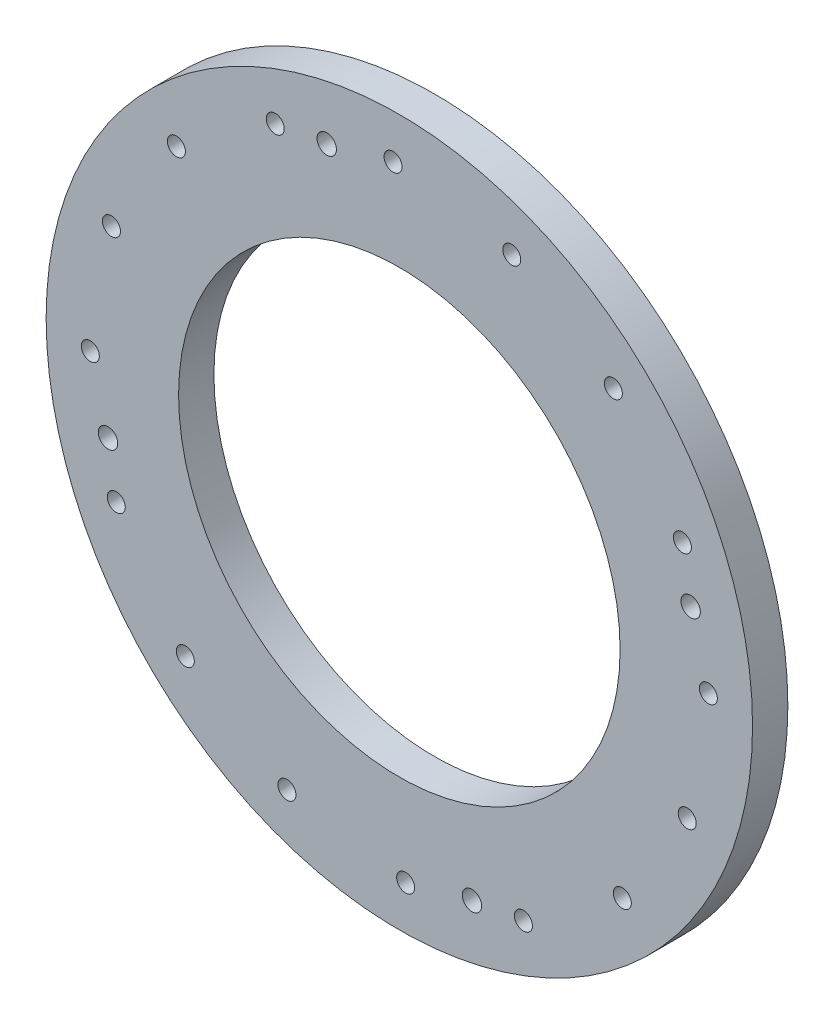
from build123d import *

# Parameters (mm, degrees)
SKETCH_1_R                = 200
EXTRUDE_1_DEPTH           = 10
SKETCH_2_R                = 125
CUT_EXTRUDE_1_DEPTH       = 284.548937575
HOLE_WIZARD_M12_1_D       = 10.2
PATTERN_CIRCULAR_1_COUNT  = 16
HOLE_WIZARD_1_D           = 11
HOLE_WIZARD_1_CBORE_D     = 18
HOLE_WIZARD_1_CBORE_DEPTH = 11
PATTERN_CIRCULAR_2_COUNT  = 4


with BuildPart() as part:
    # 草图1 → 凸台-拉伸1 (new, symmetric)
    with BuildSketch(Plane.XY):
        Circle(SKETCH_1_R)
    extrude(amount=EXTRUDE_1_DEPTH, both=True)

    # 草图2 → 切除-拉伸1 (cut, through all)
    with BuildSketch(Plane(origin=(0, 0, -10), x_dir=(-1, 0, 0), z_dir=(0, 0, -1))):
        Circle(SKETCH_2_R)
    extrude(amount=-CUT_EXTRUDE_1_DEPTH, mode=Mode.SUBTRACT)

    # M12 螺纹孔1 (through all)
    with Locations(Plane(origin=(0, 0, -10), x_dir=(-1, 0, 0), z_dir=(0, 0, -1))):
        with Locations((126.247255109, 121.188409419)):
            hole_wizard_m12_1 = Hole(HOLE_WIZARD_M12_1_D / 2)

    # 阵列(圆周)1: M12 螺纹孔1 ×16 about axis
    pattern_circular_1_axis = Axis((0, 0, 0), (0, 0, 1))
    for i in range(1, PATTERN_CIRCULAR_1_COUNT):
        add(hole_wizard_m12_1.rotate(pattern_circular_1_axis, i * 360 / PATTERN_CIRCULAR_1_COUNT), mode=Mode.SUBTRACT)

    # 打孔尺寸(%根据)内六角圆柱头螺钉的类型1 (through all)
    with Locations(Plane(origin=(0, 0, -10), x_dir=(-1, 0, 0), z_dir=(0, 0, -1))):
        with Locations((-164.950273467, 41.126722252)):
            hole_wizard_1 = CounterBoreHole(HOLE_WIZARD_1_D / 2, HOLE_WIZARD_1_CBORE_D / 2, HOLE_WIZARD_1_CBORE_DEPTH)

    # 阵列(圆周)2: 打孔尺寸(%根据)内六角圆柱头螺钉的类型1 ×4 about axis
    pattern_circular_2_axis = Axis((0, 0, 0), (0, 0, 1))
    for i in range(1, PATTERN_CIRCULAR_2_COUNT):
        add(hole_wizard_1.rotate(pattern_circular_2_axis, i * 360 / PATTERN_CIRCULAR_2_COUNT), mode=Mode.SUBTRACT)


solid = part.part
